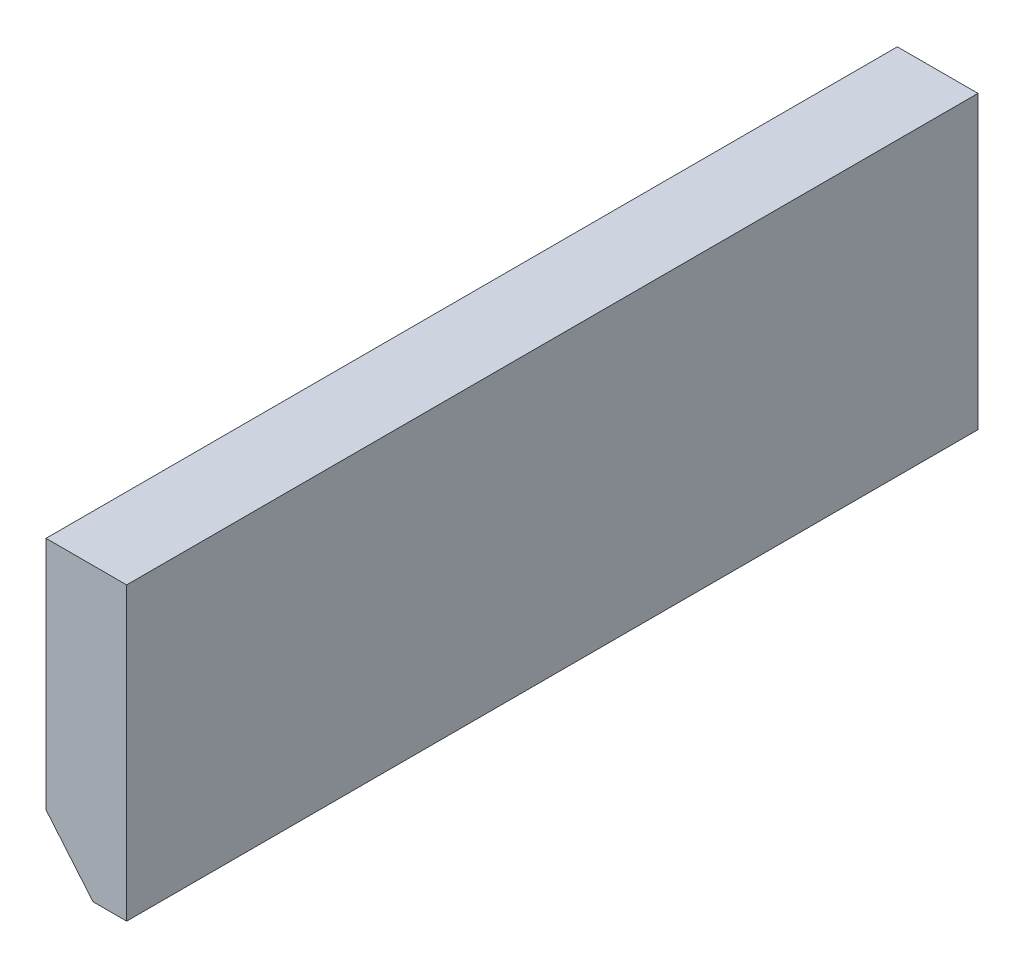
from build123d import *

# Parameters (mm, degrees)
BOSS_EXTRUDE1_DEPTH = 190


with BuildPart() as part:
    # Sketch1 → Boss-Extrude1 (new, symmetric)
    with BuildSketch(Plane.XY):
        Polygon((0, 0), (0, 130), (-36, 130), (-36, 25.026825444), (-15, 0), align=None)
    extrude(amount=BOSS_EXTRUDE1_DEPTH, both=True)


solid = part.part
